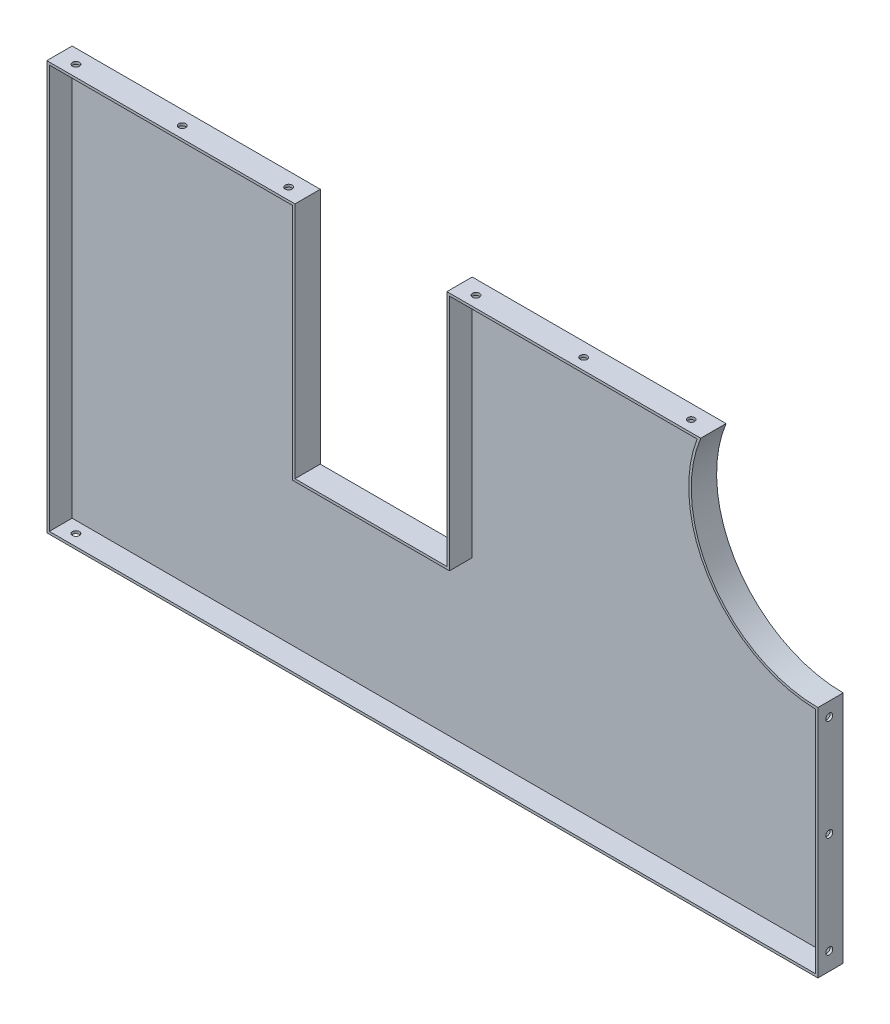
SolidWorks part; units mm, degrees
ref_plane "前视基准面" through (0, 0, 0) normal (0, 0, 1) x (1, 0, 0)
ref_plane "上视基准面" through (0, 0, 0) normal (0, 1, 0) x (1, 0, 0)
ref_plane "右视基准面" through (0, 0, 0) normal (1, 0, 0) x (0, 0, -1)
sketch "草图1" plane through (0, 0, 0) normal (0, 0, 1) x (1, 0, 0)
  line L0 (609, 0) -> (609, 357.5682) construction
  line L1 (0, 0) -> (609, 0)
  line L2 (0, 0) -> (0, 323)
  line L3 (0, 323) -> (196, 323)
  line L4 (609, 0) -> (609, 185)
  line L6 (316, 323) -> (516.5014, 323)
  line L8 (196, 323) -> (196, 135)
  line L9 (196, 135) -> (316, 135)
  line L10 (316, 323) -> (316, 135)
  arc A0 (516.5014, 323) -> (609, 185) centre (609, 285) ccw
  dimension "D3" = 285
  dimension "D7" = 100
  dimension "D1" = 323
  dimension "D2" = 609
  dimension "D4" = 120
  dimension "D5" = 188
  dimension "D6" = 196
extrude "凸台-拉伸1" add sketch "草图1" along normal blind 20
shell "抽壳1" thickness 2
sketch "草图2" plane through (0, 2, 0) normal (0, 1, 0) x (1, 0, 0)
  line L0 (2, -11) -> (116.4337, -11) construction
  line L1 (2, -20) -> (2, -2) construction
  line L2 (0, -20) -> (0, 0) construction
  circle A0 centre (14, -11) radius 2.75
  dimension "D1" = 5.5
  dimension "D2" = 14
extrude "切除-拉伸1" cut sketch "草图2" against normal blind 10 and the other way blind 338
sketch "草图3" plane through (0, 321, 0) normal (0, -1, 0) x (1, 0, 0)
  line L0 (2, 11) -> (569.7614, 11) construction
  line L1 (2, 20) -> (2, 2) construction
  line L2 (196, 20) -> (196, 0) construction
  line L3 (316, 20) -> (316, 0) construction
  circle A0 centre (98, 11) radius 2.75
  circle A1 centre (182, 11) radius 2.75
  circle A2 centre (330, 11) radius 2.75
  circle A3 centre (415, 11) radius 2.75
  circle A4 centre (500, 11) radius 2.75
  dimension "D1" = 5.5
  dimension "D2" = 5.5
  dimension "D3" = 5.5
  dimension "D4" = 5.5
  dimension "D5" = 5.5
  dimension "D6" = 14
  dimension "D7" = 84
  dimension "D8" = 14
  dimension "D9" = 85
  dimension "D10" = 85
extrude "切除-拉伸2" cut sketch "草图3" against normal blind 10
sketch "草图4" plane through (607, 0, 0) normal (-1, 0, 0) x (0, 0, 1)
  line L0 (11, 2) -> (11, 232.0985) construction
  line L1 (20, 2) -> (2, 2) construction
  line L2 (20, 0) -> (0, 0) construction
  circle A0 centre (11, 14) radius 2.75
  circle A1 centre (11, 94) radius 2.75
  circle A2 centre (11, 174) radius 2.75
  dimension "D1" = 5.5
  dimension "D2" = 5.5
  dimension "D3" = 5.5
  dimension "D4" = 80
  dimension "D5" = 80
  dimension "D6" = 14
extrude "切除-拉伸3" cut sketch "草图4" against normal blind 10
